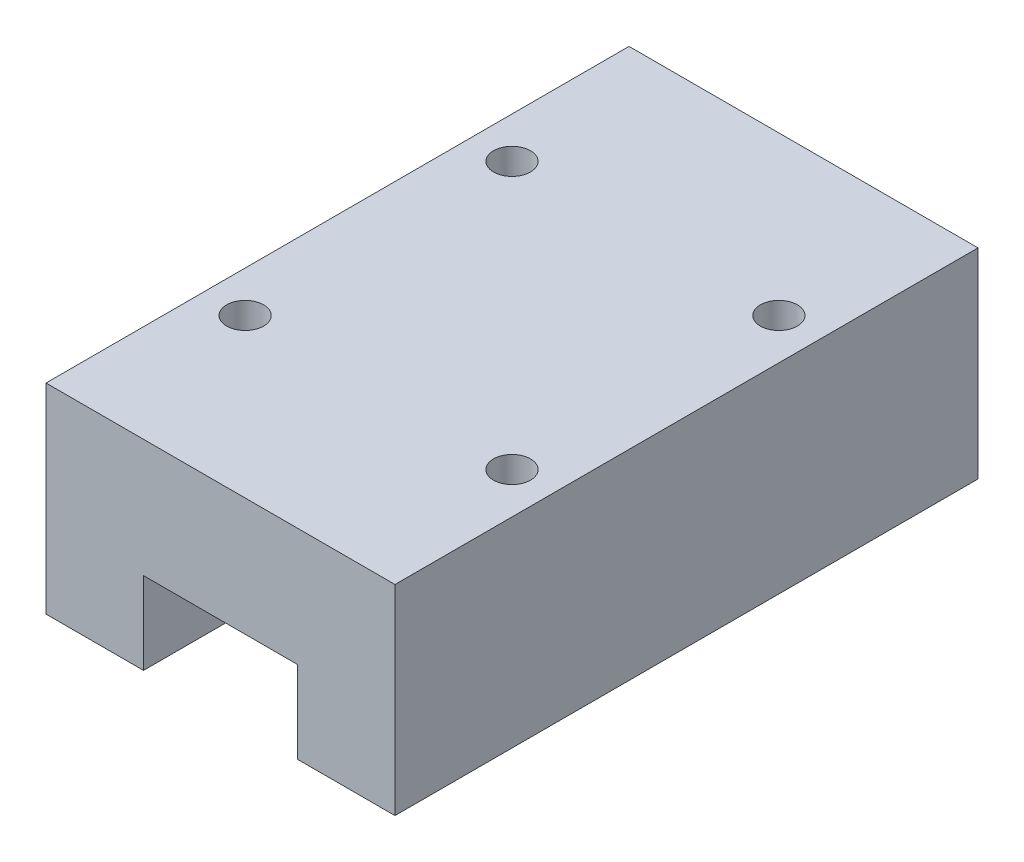
SolidWorks part; units mm, degrees
ref_plane "前视基准面" through (0, 0, 0) normal (0, 0, 1) x (1, 0, 0)
ref_plane "上视基准面" through (0, 0, 0) normal (0, 1, 0) x (1, 0, 0)
ref_plane "右视基准面" through (0, 0, 0) normal (1, 0, 0) x (0, 0, -1)
sketch "草图1" plane through (0, 0, 0) normal (0, 0, 1) x (1, 0, 0)
  line L1 (-17, 9.75) -> (17, 9.75)
  line L2 (-17, 9.75) -> (-17, -9.75)
  line L3 (-17, -9.75) -> (17, -9.75)
  line L4 (17, 9.75) -> (17, -9.75)
  line L5 (-17, 9.75) -> (17, -9.75) construction
  line L6 (-17, -9.75) -> (17, 9.75) construction
  point P0 (0, 0)
  dimension "D1" = 19.5
  dimension "D2" = 34
extrude "凸台-拉伸1" add sketch "草图1" along normal mid plane 56.8
sketch "草图2" plane through (0, 0, 0) normal (0, 0, 1) x (1, 0, 0)
  line L0 (0, 0) -> (0, -9.75) construction
  line L1 (-17, -9.75) -> (17, -9.75) construction
  line L3 (-7.5, -1.75) -> (7.5, -1.75)
  line L4 (-7.5, -1.75) -> (-7.5, -9.75)
  line L5 (-7.5, -9.75) -> (7.5, -9.75)
  line L6 (7.5, -1.75) -> (7.5, -9.75)
  line L7 (-7.5, -1.75) -> (7.5, -9.75) construction
  line L8 (-7.5, -9.75) -> (7.5, -1.75) construction
  point P5 (0, -5.75)
  dimension "D1" = 15
  dimension "D2" = 8
extrude "切除-拉伸1" cut sketch "草图2" against normal through all both and the other way through all
sketch "草图4" plane through (0, 9.75, 0) normal (0, 1, 0) x (1, 0, 0)
  line L0 (0, 28.4) -> (0, -28.4) construction
  line L1 (17, 28.4) -> (-17, 28.4) construction
  line L2 (17, -28.4) -> (-17, -28.4) construction
  line L3 (-17, 0) -> (17, 0) construction
  line L4 (-17, -28.4) -> (-17, 28.4) construction
  line L5 (17, -28.4) -> (17, 28.4) construction
  circle A0 centre (-13, 13) radius 1.8
  circle A1 centre (13, 13) radius 1.8
  circle A2 centre (13, -13) radius 1.8
  circle A3 centre (-13, -13) radius 1.8
  dimension "D2" = 3.6
  dimension "D1" = 26
  dimension "D3" = 26
extrude "切除-拉伸2" cut sketch "草图4" against normal blind 6
